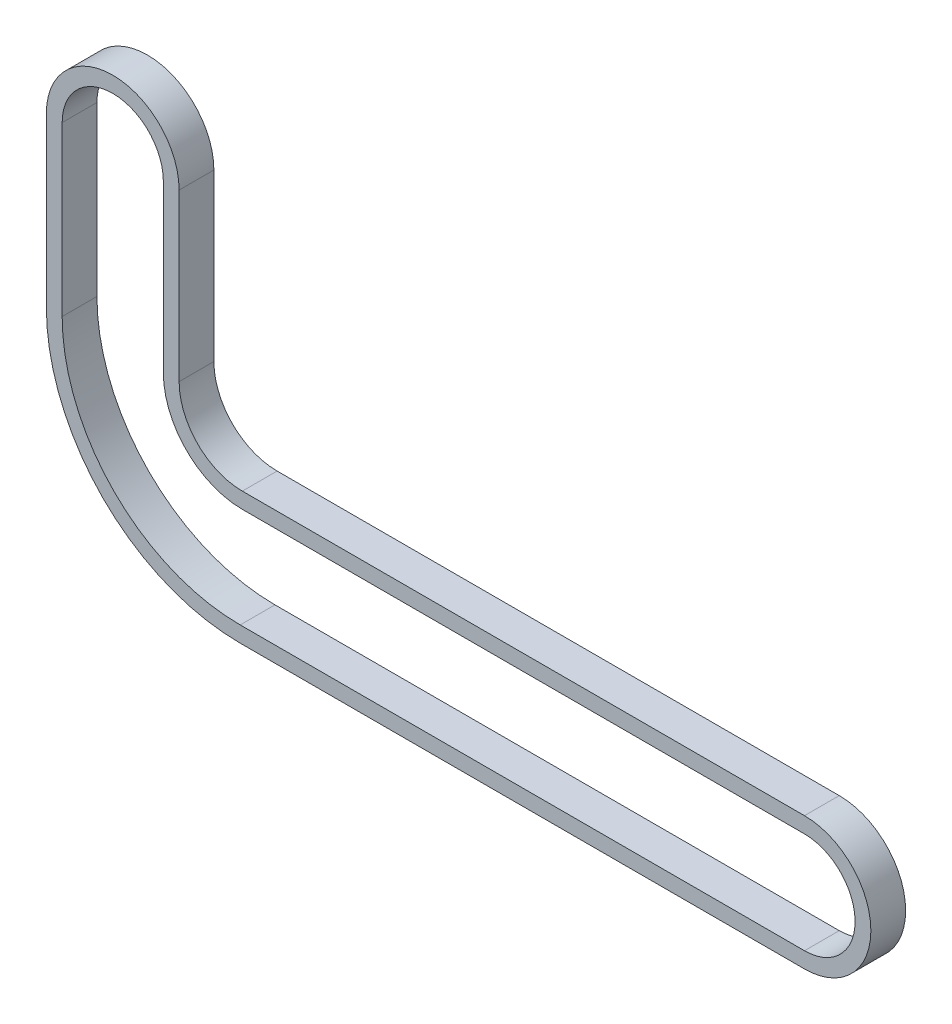
from build123d import *

# Parameters (mm, degrees)
BOSS_EXTRUDE1_DEPTH = 11


with BuildPart() as part:
    # Sketch1 → Boss-Extrude1 (new body)
    with BuildSketch(Plane.XY):
        with BuildLine():
            Line((-18.363387922, 23.381087781), (-18.363387922, 75.858020773))
            ThreePointArc((-18.363387922, 75.858020773), (-39.363387922, 96.858020773), (-60.363387922, 75.858020773))
            Line((-60.363387922, 75.858020773), (-60.363387922, 22.707373273))
            ThreePointArc((-60.363387922, 22.707373273), (-42.401334766, -20.656859064), (0.962897571, -38.618912219))
            Line((0.962897571, -38.618912219), (179.480864488, -38.618912219))
            ThreePointArc((179.480864488, -38.618912219), (200.480864488, -17.618912219), (179.480864488, 3.381087781))
            Line((179.480864488, 3.381087781), (1.636612078, 3.381087781))
            ThreePointArc((1.636612078, 3.381087781), (-12.505523546, 9.238952157), (-18.363387922, 23.381087781))
        make_face()
        with BuildLine():
            Line((-55.363387922, 75.858020773), (-55.363387922, 22.707373273))
            ThreePointArc((-55.363387922, 22.707373273), (-38.86580086, -17.121325158), (0.962897571, -33.618912219))
            Line((0.962897571, -33.618912219), (179.480864488, -33.618912219))
            ThreePointArc((179.480864488, -33.618912219), (195.480864488, -17.618912219), (179.480864488, -1.618912219))
            Line((179.480864488, -1.618912219), (1.636612078, -1.618912219))
            ThreePointArc((1.636612078, -1.618912219), (-16.041057452, 5.703418251), (-23.363387922, 23.381087781))
            Line((-23.363387922, 23.381087781), (-23.363387922, 75.858020773))
            ThreePointArc((-23.363387922, 75.858020773), (-39.363387922, 91.858020773), (-55.363387922, 75.858020773))
        make_face(mode=Mode.SUBTRACT)
    extrude(amount=-BOSS_EXTRUDE1_DEPTH)


solid = part.part
